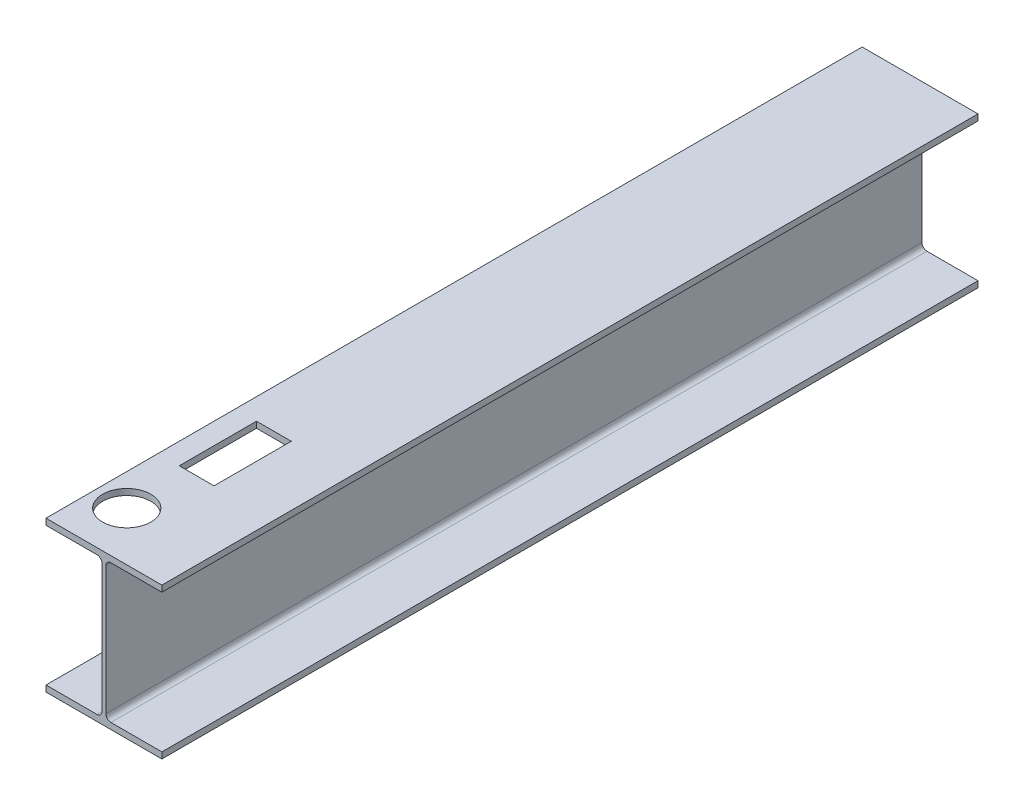
from build123d import *

# Parameters (mm, degrees)
BOSS_EXTRUDE1_DEPTH = 2113
CUT_EXTRUDE1_REACH  = 2171.532
SKETCH2_R           = 62.5
SKETCH2_W           = 90
SKETCH2_H           = 200
CUT_EXTRUDE2_REACH  = 2156.273
SKETCH3_R           = 25.5


with BuildPart() as part:
    # Sketch1 → Boss-Extrude1 (new body)
    with BuildSketch(Plane.XY):
        with BuildLine():
            Line((0, 0), (300, 0))
            Line((300, 0), (300, 16))
            Line((300, 16), (168, 16))
            ThreePointArc((168, 16), (158.807611845, 19.807611845), (155, 29))
            Line((155, 29), (155, 361))
            ThreePointArc((155, 361), (158.807611845, 370.192388155), (168, 374))
            Line((168, 374), (300, 374))
            Line((300, 374), (300, 390))
            Line((300, 390), (0, 390))
            Line((0, 390), (0, 374))
            Line((0, 374), (132, 374))
            ThreePointArc((132, 374), (141.192388155, 370.192388155), (145, 361))
            Line((145, 361), (145, 29))
            ThreePointArc((145, 29), (141.192388155, 19.807611845), (132, 16))
            Line((132, 16), (0, 16))
            Line((0, 16), (0, 0))
        make_face()
    extrude(amount=BOSS_EXTRUDE1_DEPTH)

    # Sketch2 → Cut-Extrude1 (cut, up to next)
    with BuildSketch(Plane(origin=(0, 390, 0), x_dir=(1, 0, 0), z_dir=(0, 1, 0)), mode=Mode.PRIVATE) as cut_extrude1_sk1:
        with Locations(Location((82, -1986, 0), (0, 0, 270))):
            Circle(SKETCH2_R)
    cut_extrude1_tool1 = extrude(cut_extrude1_sk1.sketch, amount=-CUT_EXTRUDE1_REACH, mode=Mode.PRIVATE) & part.part
    # Sketch2 → Cut-Extrude1 (cut, up to next)
    with BuildSketch(Plane(origin=(0, 390, 0), x_dir=(1, 0, 0), z_dir=(0, 1, 0)), mode=Mode.PRIVATE) as cut_extrude1_sk2:
        with Locations((100, -1723)):
            Rectangle(SKETCH2_W, SKETCH2_H)
    cut_extrude1_tool2 = extrude(cut_extrude1_sk2.sketch, amount=-CUT_EXTRUDE1_REACH, mode=Mode.PRIVATE) & part.part
    add(cut_extrude1_tool1.solids().sort_by_distance((82, 390, 1986))[0], mode=Mode.SUBTRACT)
    add(cut_extrude1_tool2.solids().sort_by_distance((100, 390, 1723))[0], mode=Mode.SUBTRACT)

    # Sketch3 → Cut-Extrude2 (cut, up to next)
    with BuildSketch(Plane.ZY.offset(-145), mode=Mode.PRIVATE) as cut_extrude2_sk1:
        with Locations(Location((1723, 315, 0), (0, 0, 270))):
            Circle(SKETCH3_R)
    cut_extrude2_tool1 = extrude(cut_extrude2_sk1.sketch, amount=-CUT_EXTRUDE2_REACH, mode=Mode.PRIVATE) & part.part
    add(cut_extrude2_tool1.solids().sort_by_distance((145, 315, 1723))[0], mode=Mode.SUBTRACT)


solid = part.part
